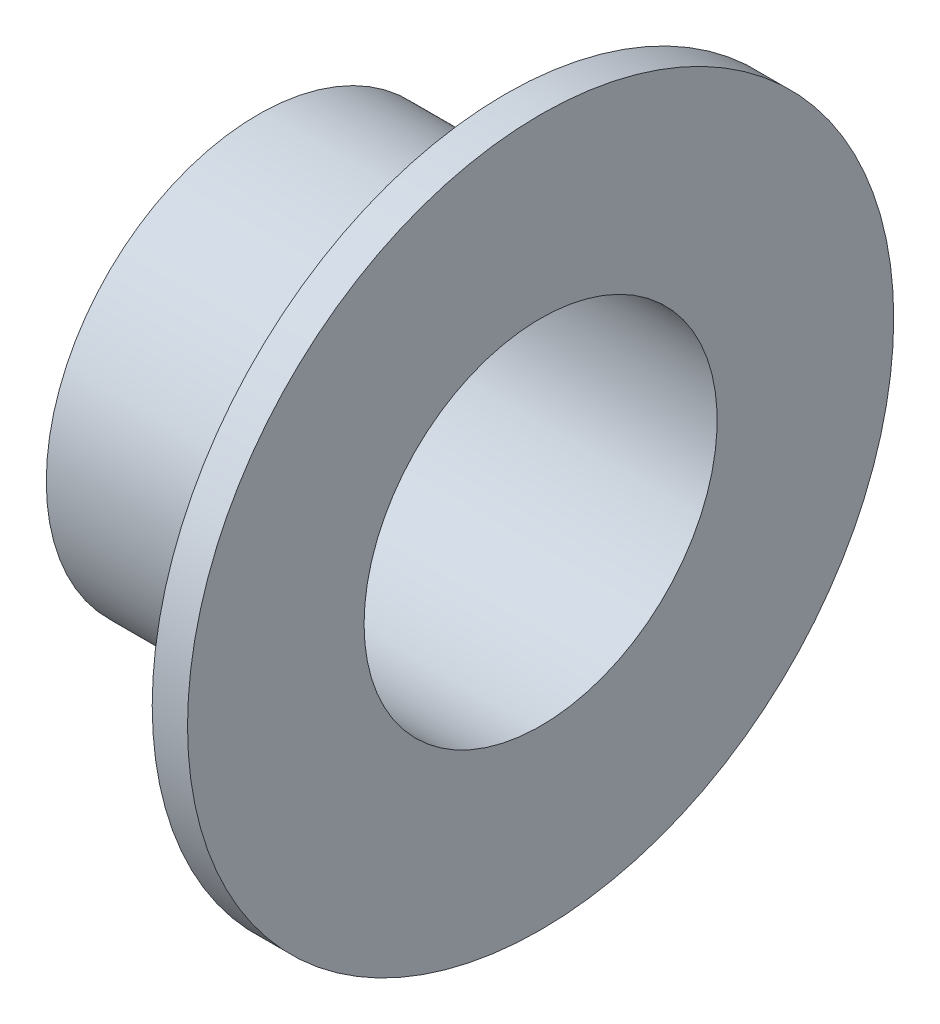
from build123d import *


with BuildPart() as part:
    # 草图1 → 旋转1 (revolve)
    with BuildSketch(Plane(origin=(0, 0, 0), x_dir=(1, 0, 0), z_dir=(0, 1, 0)), mode=Mode.PRIVATE) as revolve_1_sk:
        Polygon((0, 2.5), (0, 3), (3.5, 3), (3.5, 5), (4, 5), (4, 2.5), align=None)
    revolve(revolve_1_sk.sketch.rotate(Axis((-238.363176029, 0, 0), (1, 0, 0)), 180), axis=Axis((-238.363176029, 0, 0), (1, 0, 0)))


solid = part.part
